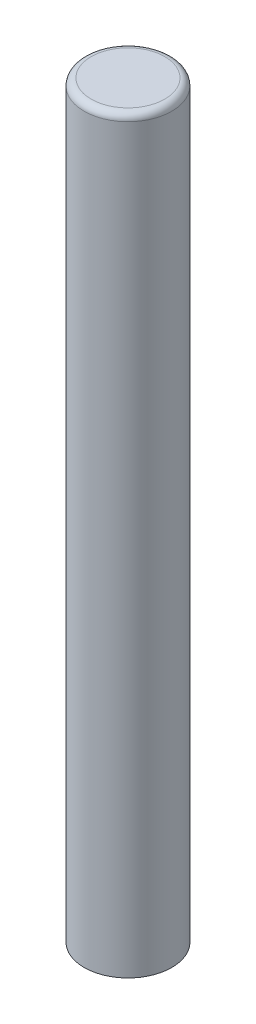
from build123d import *

# Parameters (mm, degrees)
SKETCH1_R           = 12.5
BOSS_EXTRUDE1_DEPTH = 213.5
FILLET1_R           = 2


with BuildPart() as part:
    # Sketch1 → Boss-Extrude1 (new body)
    with BuildSketch(Plane(origin=(0, 0, 0), x_dir=(1, 0, 0), z_dir=(0, 1, 0))):
        with Locations(Location((0, 0, 0), (0, 0, 270))):
            Circle(SKETCH1_R)
    extrude(amount=BOSS_EXTRUDE1_DEPTH)

    # Fillet1
    fillet1_edges = [part.edges().sort_by_distance(p)[0] for p in [
        (0, 213.5, -12.5),
    ]]
    fillet(fillet1_edges, radius=FILLET1_R)


solid = part.part
